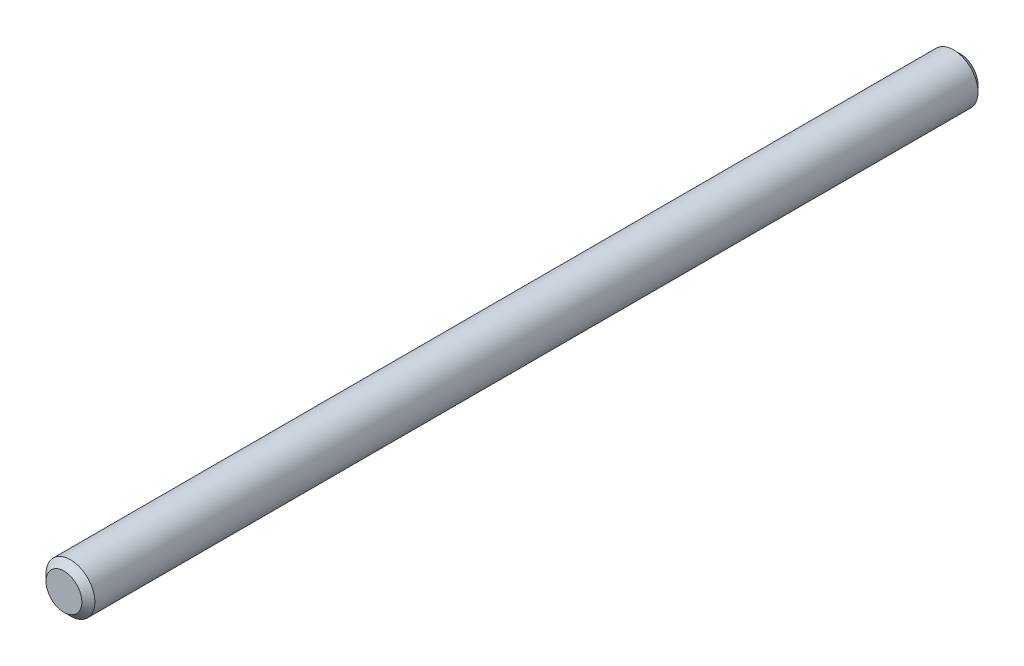
from build123d import *

# Parameters (mm, degrees)
SKETCH1_R           = 0.75
BOSS_EXTRUDE1_DEPTH = 13.75
CHAMFER1_SIZE       = 0.2


with BuildPart() as part:
    # Sketch1 → Boss-Extrude1 (new, symmetric)
    with BuildSketch(Plane.XY):
        Circle(SKETCH1_R)
    extrude(amount=BOSS_EXTRUDE1_DEPTH, both=True)

    # Chamfer1
    chamfer1_edges = [part.edges().sort_by_distance(p)[0] for p in [
        (-0.75, 0, -13.75),
        (-0.75, 0, 13.75),
    ]]
    chamfer(chamfer1_edges, length=CHAMFER1_SIZE)


solid = part.part
